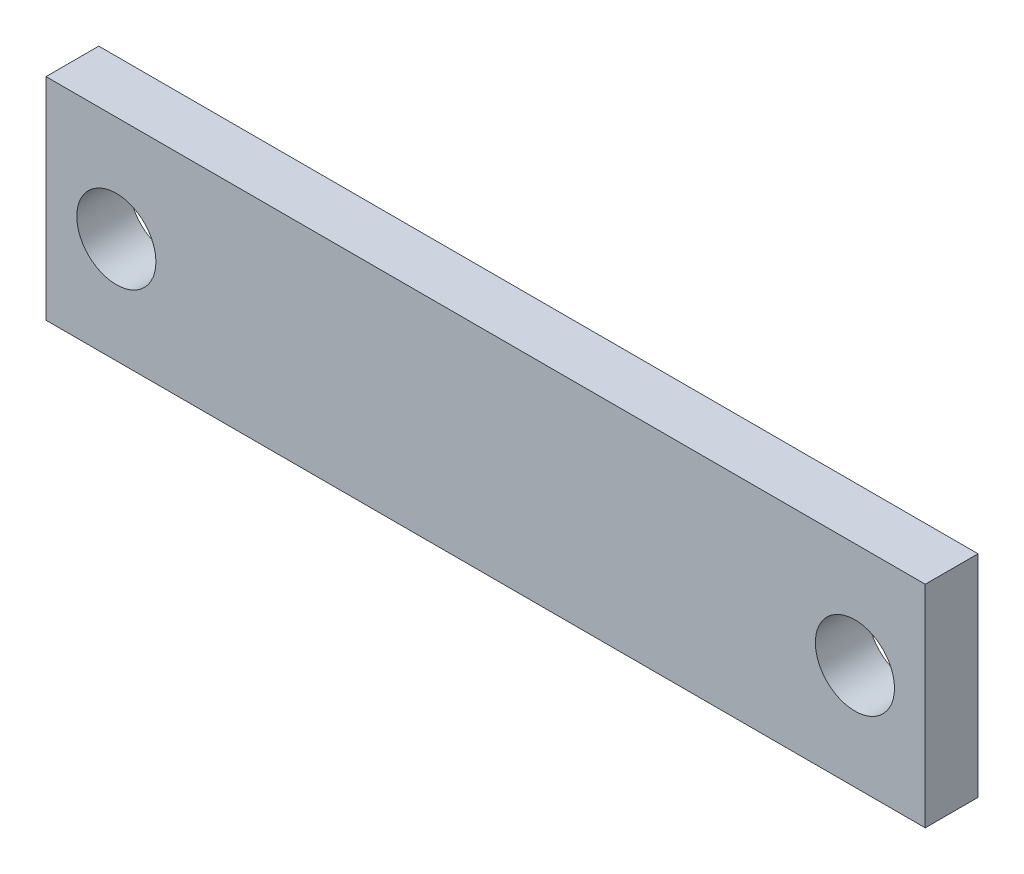
from build123d import *

# Parameters (mm, degrees)
SKETCH_1_W      = 50
SKETCH_1_H      = 12
SKETCH_1_R      = 2.25
EXTRUDE_1_DEPTH = 1.5


with BuildPart() as part:
    # 草图1 → 凸台-拉伸1 (new, symmetric)
    with BuildSketch(Plane.XY):
        Rectangle(SKETCH_1_W, SKETCH_1_H)
        with Locations((-21, 0)):
            Circle(SKETCH_1_R, mode=Mode.SUBTRACT)
        with Locations((21, 0)):
            Circle(SKETCH_1_R, mode=Mode.SUBTRACT)
    extrude(amount=EXTRUDE_1_DEPTH, both=True)


solid = part.part
